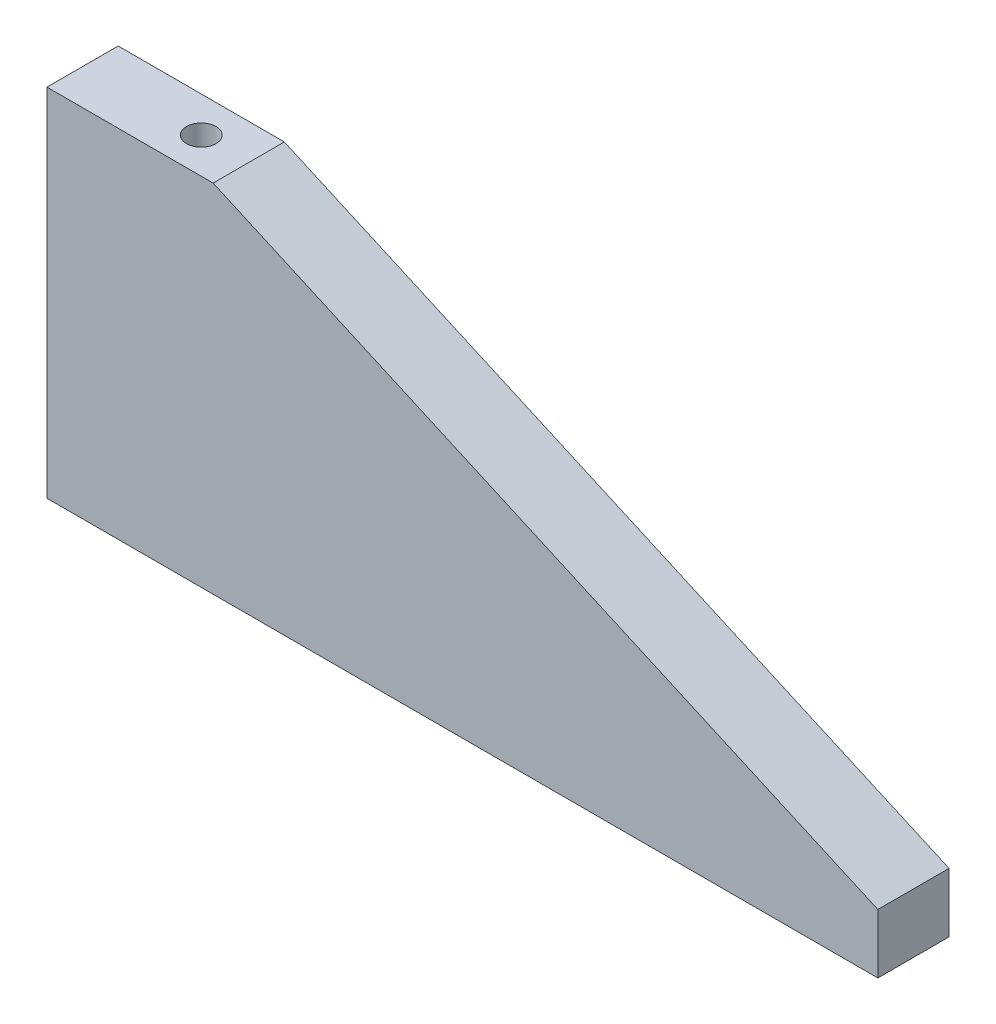
from build123d import *

# Parameters (mm, degrees)
EXTRUDE_1_DEPTH        = 12
HOLE_WIZARD_M6_1_D     = 5
HOLE_WIZARD_M6_1_DEPTH = 15
HOLE_WIZARD_M6_1_TIP   = 1.502151548
HOLE_WIZARD_M6_2_D     = 5
HOLE_WIZARD_M6_2_DEPTH = 15
HOLE_WIZARD_M6_2_TIP   = 1.502151548
HOLE_WIZARD_M6_3_D     = 5
HOLE_WIZARD_M6_3_DEPTH = 15
HOLE_WIZARD_M6_3_TIP   = 1.502151548


with BuildPart() as part:
    # 草图1 → 凸台-拉伸1 (new body)
    with BuildSketch(Plane.XY):
        Polygon((0, 0), (0, -60), (140, -60), (140, -50), (28, 0), align=None)
    extrude(amount=EXTRUDE_1_DEPTH)

    # M6 螺纹孔1
    with Locations(Plane.ZY):
        with Locations((6, -15), (6, -45)):
            Hole(HOLE_WIZARD_M6_1_D / 2, depth=HOLE_WIZARD_M6_1_DEPTH)
            with Locations((0, 0, -(HOLE_WIZARD_M6_1_DEPTH + HOLE_WIZARD_M6_1_TIP / 2))):  # 118° drill point
                Cone(0, HOLE_WIZARD_M6_1_D / 2, HOLE_WIZARD_M6_1_TIP, mode=Mode.SUBTRACT)

    # M6 螺纹孔2
    with Locations(Plane(origin=(0, -60, 0), x_dir=(-1, 0, 0), z_dir=(0, -1, 0))):
        with Locations((-120, -6), (-20, -6)):
            Hole(HOLE_WIZARD_M6_2_D / 2, depth=HOLE_WIZARD_M6_2_DEPTH)
            with Locations((0, 0, -(HOLE_WIZARD_M6_2_DEPTH + HOLE_WIZARD_M6_2_TIP / 2))):  # 118° drill point
                Cone(0, HOLE_WIZARD_M6_2_D / 2, HOLE_WIZARD_M6_2_TIP, mode=Mode.SUBTRACT)

    # M6 螺纹孔3
    with Locations(Plane(origin=(0, 0, 0), x_dir=(1, 0, 0), z_dir=(0, 1, 0))):
        with Locations((20, -6)):
            Hole(HOLE_WIZARD_M6_3_D / 2, depth=HOLE_WIZARD_M6_3_DEPTH)
            with Locations((0, 0, -(HOLE_WIZARD_M6_3_DEPTH + HOLE_WIZARD_M6_3_TIP / 2))):  # 118° drill point
                Cone(0, HOLE_WIZARD_M6_3_D / 2, HOLE_WIZARD_M6_3_TIP, mode=Mode.SUBTRACT)


solid = part.part
